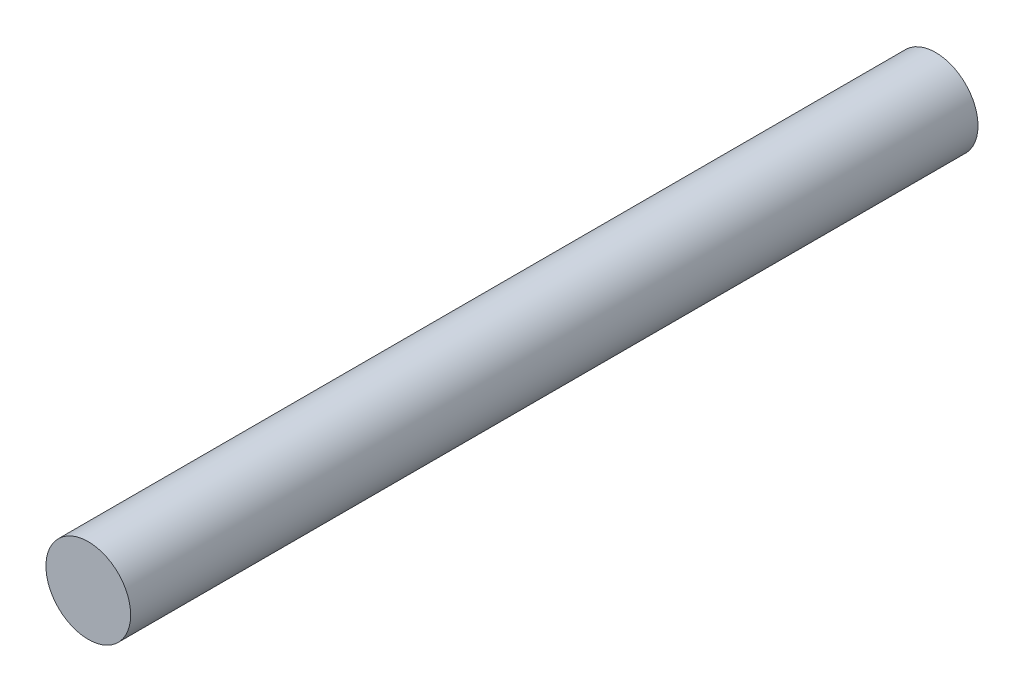
from build123d import *

# Parameters (mm, degrees)
SKETCH1_R           = 2.5
BOSS_EXTRUDE1_DEPTH = 50


with BuildPart() as part:
    # Sketch1 → Boss-Extrude1 (new body)
    with BuildSketch(Plane.XY):
        Circle(SKETCH1_R)
    extrude(amount=BOSS_EXTRUDE1_DEPTH)


solid = part.part
